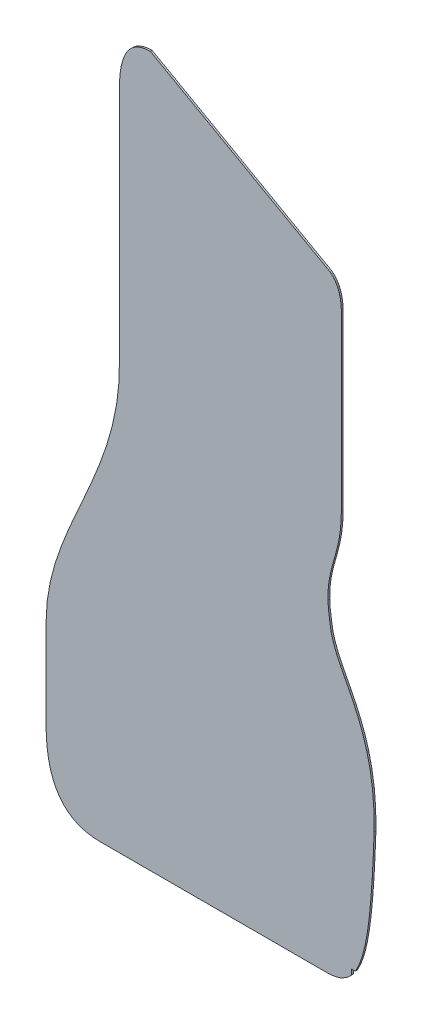
SolidWorks part; units mm, degrees
ref_plane "前视基准面" through (0, 0, 0) normal (0, 0, 1) x (1, 0, 0)
ref_plane "上视基准面" through (0, 0, 0) normal (0, 1, 0) x (1, 0, 0)
ref_plane "右视基准面" through (0, 0, 0) normal (1, 0, 0) x (0, 0, -1)
other "Configuration Table"
sketch "草图1" plane through (0, 0, 0) normal (0, 0, 1) x (1, 0, 0)
  line L0 (103, 235) -> (-24.8333, 235)
  line L1 (-24.8333, 235) -> (-152.6667, 235)
  line L2 (-152.6667, 235) -> (-280.5, 235)
  line L3 (-280.5, 235) -> (-293.0357, 235.6378)
  line L4 (-293.0357, 235.6378) -> (-304.6429, 237.551)
  line L5 (-304.6429, 237.551) -> (-315.3214, 240.7398)
  line L6 (-315.3214, 240.7398) -> (-325.0714, 245.2041)
  line L7 (-325.0714, 245.2041) -> (-333.8929, 250.9439)
  line L8 (-333.8929, 250.9439) -> (-341.7857, 257.9592)
  line L9 (-341.7857, 257.9592) -> (-348.75, 266.25)
  line L10 (-348.75, 266.25) -> (-354.7857, 275.8163)
  line L11 (-354.7857, 275.8163) -> (-359.8929, 286.6582)
  line L12 (-359.8929, 286.6582) -> (-364.0714, 298.7755)
  line L13 (-364.0714, 298.7755) -> (-367.3214, 312.1684)
  line L14 (-367.3214, 312.1684) -> (-369.6429, 326.8367)
  line L15 (-369.6429, 326.8367) -> (-371.0357, 342.7806)
  line L16 (-371.0357, 342.7806) -> (-371.5, 360)
  line L17 (-371.5, 360) -> (-371.5, 410)
  line L18 (-371.5, 410) -> (-371.5, 460)
  line L19 (-371.5, 460) -> (-371.5, 510)
  line L20 (-371.5, 510) -> (-369.6073, 541.7165)
  line L21 (-369.6073, 541.7165) -> (-364.3178, 572.7114)
  line L22 (-364.3178, 572.7114) -> (-356.2141, 603.1815)
  line L23 (-356.2141, 603.1815) -> (-345.879, 633.3236)
  line L24 (-345.879, 633.3236) -> (-333.8952, 663.3345)
  line L25 (-333.8952, 663.3345) -> (-320.8455, 693.4111)
  line L26 (-320.8455, 693.4111) -> (-307.3125, 723.75)
  line L27 (-307.3125, 723.75) -> (-293.879, 754.5481)
  line L28 (-293.879, 754.5481) -> (-281.1277, 786.0022)
  line L29 (-281.1277, 786.0022) -> (-269.6414, 818.309)
  line L30 (-269.6414, 818.309) -> (-260.0027, 851.6655)
  line L31 (-260.0027, 851.6655) -> (-252.7945, 886.2682)
  line L32 (-252.7945, 886.2682) -> (-248.5993, 922.3141)
  line L33 (-248.5993, 922.3141) -> (-248, 960)
  line L34 (-248, 960) -> (-248, 1090)
  line L35 (-248, 1090) -> (-248, 1220)
  line L36 (-248, 1220) -> (-248, 1350)
  line L37 (-248, 1350) -> (-247.7347, 1361.0204)
  line L38 (-247.7347, 1361.0204) -> (-246.9388, 1371.2245)
  line L39 (-246.9388, 1371.2245) -> (-245.6122, 1380.6122)
  line L40 (-245.6122, 1380.6122) -> (-243.7551, 1389.1837)
  line L41 (-243.7551, 1389.1837) -> (-241.3673, 1396.9388)
  line L42 (-241.3673, 1396.9388) -> (-238.449, 1403.8776)
  line L43 (-238.449, 1403.8776) -> (-235, 1410)
  line L44 (-235, 1410) -> (-231.0204, 1415.3061)
  line L45 (-231.0204, 1415.3061) -> (-226.5102, 1419.7959)
  line L46 (-226.5102, 1419.7959) -> (-221.4694, 1423.4694)
  line L47 (-221.4694, 1423.4694) -> (-215.898, 1426.3265)
  line L48 (-215.898, 1426.3265) -> (-209.7959, 1428.3673)
  line L49 (-209.7959, 1428.3673) -> (-203.1633, 1429.5918)
  line L50 (-203.1633, 1429.5918) -> (-196, 1430)
  line L51 (-196, 1430) -> (-95.25, 1373.3333)
  line L52 (-95.25, 1373.3333) -> (5.5, 1316.6667)
  line L53 (5.5, 1316.6667) -> (106.25, 1260)
  line L54 (106.25, 1260) -> (108.9362, 1257.8878)
  line L55 (108.9362, 1257.8878) -> (111.4235, 1255.551)
  line L56 (111.4235, 1255.551) -> (113.7117, 1252.9898)
  line L57 (113.7117, 1252.9898) -> (115.801, 1250.2041)
  line L58 (115.801, 1250.2041) -> (117.6913, 1247.1939)
  line L59 (117.6913, 1247.1939) -> (119.3827, 1243.9592)
  line L60 (119.3827, 1243.9592) -> (120.875, 1240.5)
  line L61 (120.875, 1240.5) -> (122.1684, 1236.8163)
  line L62 (122.1684, 1236.8163) -> (123.2628, 1232.9082)
  line L63 (123.2628, 1232.9082) -> (124.1582, 1228.7755)
  line L64 (124.1582, 1228.7755) -> (124.8546, 1224.4184)
  line L65 (124.8546, 1224.4184) -> (125.352, 1219.8367)
  line L66 (125.352, 1219.8367) -> (125.6505, 1215.0306)
  line L67 (125.6505, 1215.0306) -> (125.75, 1210)
  line L68 (125.75, 1210) -> (125.75, 1113.3333)
  line L69 (125.75, 1113.3333) -> (125.75, 1016.6667)
  line L70 (125.75, 1016.6667) -> (125.75, 920)
  line L71 (125.75, 920) -> (125.281, 904.7303)
  line L72 (125.281, 904.7303) -> (123.9876, 890.9038)
  line L73 (123.9876, 890.9038) -> (122.0405, 878.2799)
  line L74 (122.0405, 878.2799) -> (119.6101, 866.6181)
  line L75 (119.6101, 866.6181) -> (116.867, 855.6778)
  line L76 (116.867, 855.6778) -> (113.9818, 845.2187)
  line L77 (113.9818, 845.2187) -> (111.125, 835)
  line L78 (111.125, 835) -> (108.4672, 824.7813)
  line L79 (108.4672, 824.7813) -> (106.1789, 814.3222)
  line L80 (106.1789, 814.3222) -> (104.4308, 803.3819)
  line L81 (104.4308, 803.3819) -> (103.3932, 791.7201)
  line L82 (103.3932, 791.7201) -> (103.2369, 779.0962)
  line L83 (103.2369, 779.0962) -> (104.1323, 765.2697)
  line L84 (104.1323, 765.2697) -> (106.25, 750)
  line L85 (106.25, 750) -> (108.5868, 735.4045)
  line L86 (108.5868, 735.4045) -> (112.6079, 721.3994)
  line L87 (112.6079, 721.3994) -> (118.0076, 707.6567)
  line L88 (118.0076, 707.6567) -> (124.4803, 693.8484)
  line L89 (124.4803, 693.8484) -> (131.7206, 679.6465)
  line L90 (131.7206, 679.6465) -> (139.4227, 664.723)
  line L91 (139.4227, 664.723) -> (147.2812, 648.75)
  line L92 (147.2812, 648.75) -> (154.9905, 631.3994)
  line L93 (154.9905, 631.3994) -> (162.245, 612.3433)
  line L94 (162.245, 612.3433) -> (168.7391, 591.2536)
  line L95 (168.7391, 591.2536) -> (174.1672, 567.8025)
  line L96 (174.1672, 567.8025) -> (178.2238, 541.6618)
  line L97 (178.2238, 541.6618) -> (180.6032, 512.5036)
  line L98 (180.6032, 512.5036) -> (181, 480)
  line L99 (181, 480) -> (179.4934, 443.1706)
  line L100 (179.4934, 443.1706) -> (177.7026, 409.7522)
  line L101 (177.7026, 409.7522) -> (175.5423, 379.6356)
  line L102 (175.5423, 379.6356) -> (172.9271, 352.7114)
  line L103 (172.9271, 352.7114) -> (169.7719, 328.8703)
  line L104 (169.7719, 328.8703) -> (165.9913, 308.0029)
  line L105 (165.9913, 308.0029) -> (161.5, 290)
  line L106 (161.5, 290) -> (156.2128, 274.7522)
  line L107 (156.2128, 274.7522) -> (150.0445, 262.1501)
  line L108 (150.0445, 262.1501) -> (142.9096, 252.0845)
  line L109 (142.9096, 252.0845) -> (134.723, 244.4461)
  line L110 (134.723, 244.4461) -> (125.3994, 239.1254)
  line L111 (125.3994, 239.1254) -> (114.8535, 236.0131)
  line L112 (114.8535, 236.0131) -> (103, 235)
  point P0 (0, 0)
  dimension "D1" = 0.4643
  dimension "D2" = 1.8571
  dimension "D3" = 1.8927
  dimension "D4" = 4.1786
  dimension "D5" = 7.1822
  dimension "D6" = 7.4286
  dimension "D7" = 11.6071
  dimension "D8" = 15.2859
  dimension "D9" = 16.7143
  dimension "D10" = 22.75
  dimension "D11" = 25.621
  dimension "D12" = 29.7143
  dimension "D13" = 37.6048
  dimension "D14" = 37.6071
  dimension "D15" = 46.4286
  dimension "D16" = 50.6545
  dimension "D17" = 56.1786
  dimension "D18" = 64.1875
  dimension "D19" = 66.8571
  dimension "D20" = 77.621
  dimension "D21" = 78.4643
  dimension "D22" = 90.3723
  dimension "D23" = 91
  dimension "D24" = 101.8586
  dimension "D25" = 111.4973
  dimension "D26" = 118.7055
  dimension "D27" = 122.9007
  dimension "D28" = 123.5
  dimension "D29" = 123.7653
  dimension "D30" = 124.5612
  dimension "D31" = 125.8878
  dimension "D32" = 127.7449
  dimension "D33" = 130.1327
  dimension "D34" = 133.051
  dimension "D35" = 136.5
  dimension "D36" = 140.4796
  dimension "D37" = 144.9898
  dimension "D38" = 150.0306
  dimension "D39" = 155.602
  dimension "D40" = 161.7041
  dimension "D41" = 168.3367
  dimension "D42" = 175.5
  dimension "D43" = 218.8333
  dimension "D44" = 276.25
  dimension "D45" = 346.6667
  dimension "D46" = 371.5
  dimension "D47" = 377
  dimension "D48" = 474.5
  dimension "D49" = 474.7369
  dimension "D50" = 474.8932
  dimension "D51" = 475.6323
  dimension "D52" = 475.9308
  dimension "D53" = 477.6789
  dimension "D54" = 477.75
  dimension "D55" = 479.9672
  dimension "D56" = 480.0868
  dimension "D57" = 480.4362
  dimension "D58" = 482.625
  dimension "D59" = 482.9235
  dimension "D60" = 484.1079
  dimension "D61" = 485.2117
  dimension "D62" = 485.4818
  dimension "D63" = 486.3535
  dimension "D64" = 487.301
  dimension "D65" = 488.367
  dimension "D66" = 489.1913
  dimension "D67" = 489.5076
  dimension "D68" = 490.8827
  dimension "D69" = 491.1101
  dimension "D70" = 492.375
  dimension "D71" = 493.5405
  dimension "D72" = 493.6684
  dimension "D73" = 494.7628
  dimension "D74" = 495.4876
  dimension "D75" = 495.6582
  dimension "D76" = 495.9803
  dimension "D77" = 496.3546
  dimension "D78" = 496.781
  dimension "D79" = 496.852
  dimension "D80" = 496.8994
  dimension "D81" = 497.1505
  dimension "D82" = 497.25
  dimension "D83" = 503.2206
  dimension "D84" = 506.223
  dimension "D85" = 510.9227
  dimension "D86" = 514.4096
  dimension "D87" = 518.7812
  dimension "D88" = 521.5445
  dimension "D89" = 526.4905
  dimension "D90" = 527.7128
  dimension "D91" = 533
  dimension "D92" = 533.745
  dimension "D93" = 537.4913
  dimension "D94" = 540.2391
  dimension "D95" = 541.2719
  dimension "D96" = 544.4271
  dimension "D97" = 545.6672
  dimension "D98" = 547.0423
  dimension "D99" = 549.2026
  dimension "D100" = 549.7238
  dimension "D101" = 550.9934
  dimension "D102" = 552.1032
  dimension "D103" = 552.5
  dimension "D104" = 0.6378
  dimension "D105" = 1.0131
  dimension "D106" = 2.551
  dimension "D107" = 4.1254
  dimension "D108" = 5.7398
  dimension "D109" = 9.4461
  dimension "D110" = 10.2041
  dimension "D111" = 15.9439
  dimension "D112" = 17.0845
  dimension "D113" = 22.9592
  dimension "D114" = 27.1501
  dimension "D115" = 31.25
  dimension "D116" = 39.7522
  dimension "D117" = 40.8163
  dimension "D118" = 51.6582
  dimension "D119" = 55
  dimension "D120" = 63.7755
  dimension "D121" = 73.0029
  dimension "D122" = 77.1684
  dimension "D123" = 91.8367
  dimension "D124" = 93.8703
  dimension "D125" = 107.7806
  dimension "D126" = 117.7114
  dimension "D127" = 125
  dimension "D128" = 144.6356
  dimension "D129" = 174.7522
  dimension "D130" = 175
  dimension "D131" = 208.1706
  dimension "D132" = 225
  dimension "D133" = 245
  dimension "D134" = 275
  dimension "D135" = 277.5036
  dimension "D136" = 306.6618
  dimension "D137" = 306.7165
  dimension "D138" = 332.8025
  dimension "D139" = 337.7114
  dimension "D140" = 356.2536
  dimension "D141" = 368.1815
  dimension "D142" = 377.3433
  dimension "D143" = 396.3994
  dimension "D144" = 398.3236
  dimension "D145" = 413.75
  dimension "D146" = 428.3345
  dimension "D147" = 429.723
  dimension "D148" = 444.6465
  dimension "D149" = 458.4111
  dimension "D150" = 458.8484
  dimension "D151" = 472.6567
  dimension "D152" = 486.3994
  dimension "D153" = 488.75
  dimension "D154" = 500.4045
  dimension "D155" = 515
  dimension "D156" = 519.5481
  dimension "D157" = 530.2697
  dimension "D158" = 544.0962
  dimension "D159" = 551.0022
  dimension "D160" = 556.7201
  dimension "D161" = 568.3819
  dimension "D162" = 579.3222
  dimension "D163" = 583.309
  dimension "D164" = 589.7813
  dimension "D165" = 600
  dimension "D166" = 610.2187
  dimension "D167" = 616.6655
  dimension "D168" = 620.6778
  dimension "D169" = 631.6181
  dimension "D170" = 643.2799
  dimension "D171" = 651.2682
  dimension "D172" = 655.9038
  dimension "D173" = 669.7303
  dimension "D174" = 685
  dimension "D175" = 687.3141
  dimension "D176" = 725
  dimension "D177" = 781.6667
  dimension "D178" = 855
  dimension "D179" = 878.3333
  dimension "D180" = 975
  dimension "D181" = 980.0306
  dimension "D182" = 984.8367
  dimension "D183" = 985
  dimension "D184" = 989.4184
  dimension "D185" = 993.7755
  dimension "D186" = 997.9082
  dimension "D187" = 1001.8163
  dimension "D188" = 1005.5
  dimension "D189" = 1008.9592
  dimension "D190" = 1012.1939
  dimension "D191" = 1015.2041
  dimension "D192" = 1017.9898
  dimension "D193" = 1020.551
  dimension "D194" = 1022.8878
  dimension "D195" = 1025
  dimension "D196" = 1081.6667
  dimension "D197" = 1115
  dimension "D198" = 1126.0204
  dimension "D199" = 1136.2245
  dimension "D200" = 235
  dimension "D201" = 1145.6122
  dimension "D202" = 1154.1837
  dimension "D203" = 1161.9388
  dimension "D204" = 1168.8776
  dimension "D205" = 1175
  dimension "D206" = 1180.3061
  dimension "D207" = 1184.7959
  dimension "D208" = 1188.4694
  dimension "D209" = 1191.3265
  dimension "D210" = 1193.3673
  dimension "D211" = 1194.5918
extrude "凸台-拉伸1" add sketch "草图1" against normal mid plane 3
sketch "草图2" plane through (0, 0, 0) normal (0, 0, 1) x (1, 0, 0)
  line L0 (143, 239) -> (175, 239)
  line L1 (175, 239) -> (175, 261)
  line L2 (175, 261) -> (143, 261)
  line L3 (143, 261) -> (143, 239)
  line L4 (143, 1139) -> (175, 1139)
  line L5 (175, 1139) -> (175, 1161)
  line L6 (175, 1161) -> (143, 1161)
  line L7 (143, 1161) -> (143, 1139)
  point P0 (0, 0)
  dimension "D1" = 32
  dimension "D2" = 175
  dimension "D3" = 22
  dimension "D4" = 900
  dimension "D5" = 922
  dimension "D6" = 1161
extrude "切除-拉伸1" cut sketch "草图2" against normal mid plane 20
